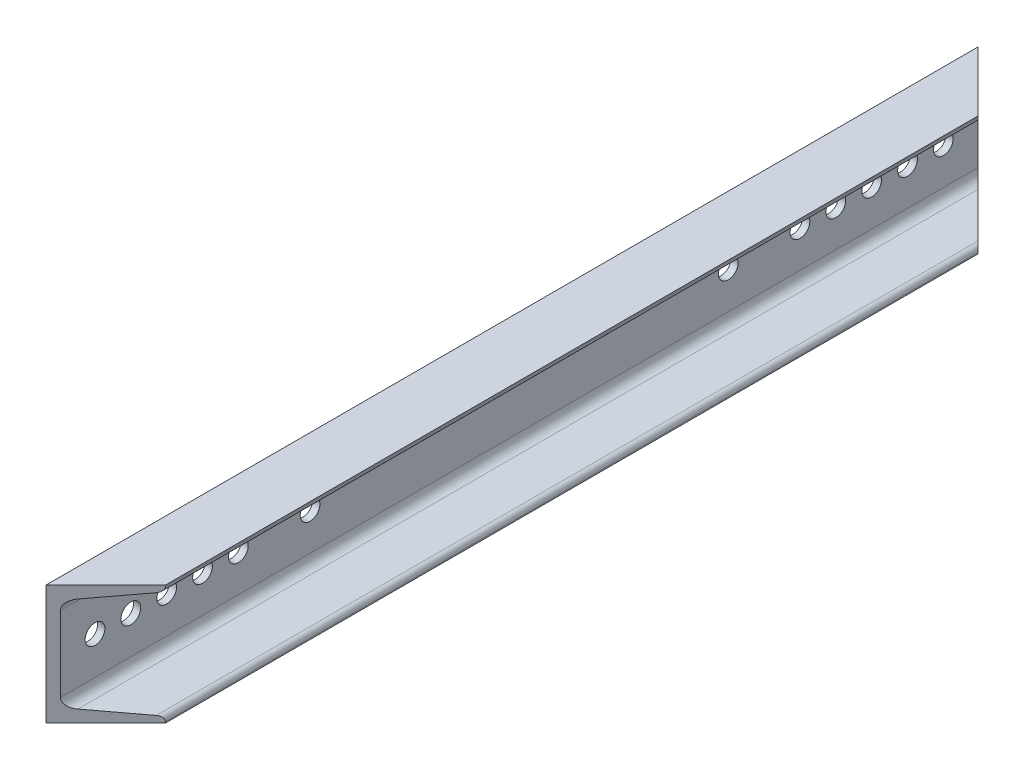
SolidWorks part; units mm, degrees
material "1023 carbon steel plate (SS)"
ref_plane "Front Plane" through (0, 0, 0) normal (0, 0, 1) x (1, 0, 0)
ref_plane "Top Plane" through (0, 0, 0) normal (0, 1, 0) x (1, 0, 0)
ref_plane "Right Plane" through (0, 0, 0) normal (1, 0, 0) x (0, 0, -1)
sketch "Sketch1" plane through (0, 0, 0) normal (0, 0, 1) x (1, 0, 0)
  line L0 (0, 0) -> (0, -100)
  line L1 (0, -100) -> (50, -100)
  line L2 (0, 0) -> (50, 0)
  line L3 (50, 0) -> (50, -1.0747)
  line L4 (50, -100) -> (50, -98.9253)
  line L5 (46.1263, -5.5309) -> (13.317, -10.1419)
  line L6 (6, -18.5592) -> (6, -81.4408)
  line L7 (13.317, -89.8581) -> (46.1263, -94.4691)
  line L8 (25, 0) -> (25, -8.5) construction
  line L9 (25, -100) -> (25, -91.5) construction
  arc A0 (6, -81.4408) -> (13.317, -89.8581) centre (14.5, -81.4408) ccw
  arc A1 (13.317, -10.1419) -> (6, -18.5592) centre (14.5, -18.5592) ccw
  arc A2 (50, -98.9253) -> (46.1263, -94.4691) centre (45.5, -98.9253) ccw
  arc A3 (50, -1.0747) -> (46.1263, -5.5309) centre (45.5, -1.0747) cw
  dimension "D8" = 8.5
  dimension "D9" = 4.5
  dimension "D1" = 100
  dimension "D2" = 50
  dimension "D3" = 50
  dimension "D4" = 6
  dimension "D5" = 8.5
  dimension "D6" = 8.5
  dimension "D7" = 98
extrude "Boss-Extrude1" add sketch "Sketch1" along normal blind 1000
sketch "Sketch5" plane through (0, 0, 0) normal (0, 1, 0) x (1, 0, 0)
  line L0 (0, -111.1923) -> (155.0079, -266.2002)
  line L1 (155.0079, -266.2002) -> (155.0079, 58.5188)
  line L3 (0, -1000) -> (0, 0) construction
  line L4 (197.3989, -693.7934) -> (279.116, -1211.0703)
  line L5 (197.3989, -693.7934) -> (0, -891.1923)
  line L8 (155.0079, 58.5188) -> (-221.0104, 43.9259)
  line L9 (-221.0104, 43.9259) -> (0, -111.1923)
  line L10 (279.116, -1211.0703) -> (0, -1168.3519)
  line L11 (0, -1168.3519) -> (-115.4003, -952.4318)
  line L12 (-115.4003, -952.4318) -> (0, -891.1923)
  dimension "D1" = 45
  dimension "D2" = 45
  dimension "D3" = 780
extrude "Cut-Extrude4" cut sketch "Sketch5" against normal blind 100
sketch "Sketch6" plane through (0, 0, 0) normal (-1, 0, 0) x (0, 0, 1)
  line L0 (111.1923, -100) -> (111.1923, 0) construction
  line L1 (891.1923, -100) -> (111.1923, -100) construction
  line L2 (501.1923, 0) -> (501.1923, -45.1438) construction
  line L3 (891.1923, 0) -> (111.1923, 0) construction
  circle A0 centre (146.1923, -50) radius 8.25
  circle A1 centre (176.1923, -50) radius 8.25
  circle A2 centre (206.1923, -50) radius 8.25
  circle A3 centre (236.1923, -50) radius 8.25
  circle A4 centre (266.1923, -50) radius 8.25
  circle A5 centre (326.1923, -50) radius 8.25
  circle A6 centre (676.1923, -50) radius 8.25
  circle A7 centre (736.1923, -50) radius 8.25
  circle A8 centre (766.1923, -50) radius 8.25
  circle A9 centre (796.1923, -50) radius 8.25
  circle A10 centre (826.1923, -50) radius 8.25
  circle A11 centre (856.1923, -50) radius 8.25
  dimension "D1" = 35
  dimension "D2" = 30
  dimension "D3" = 30
  dimension "D4" = 30
  dimension "D5" = 30
  dimension "D6" = 60
  dimension "D7" = 16.5
  dimension "D8" = 50
extrude "Cut-Extrude5" cut sketch "Sketch6" against normal blind 100
